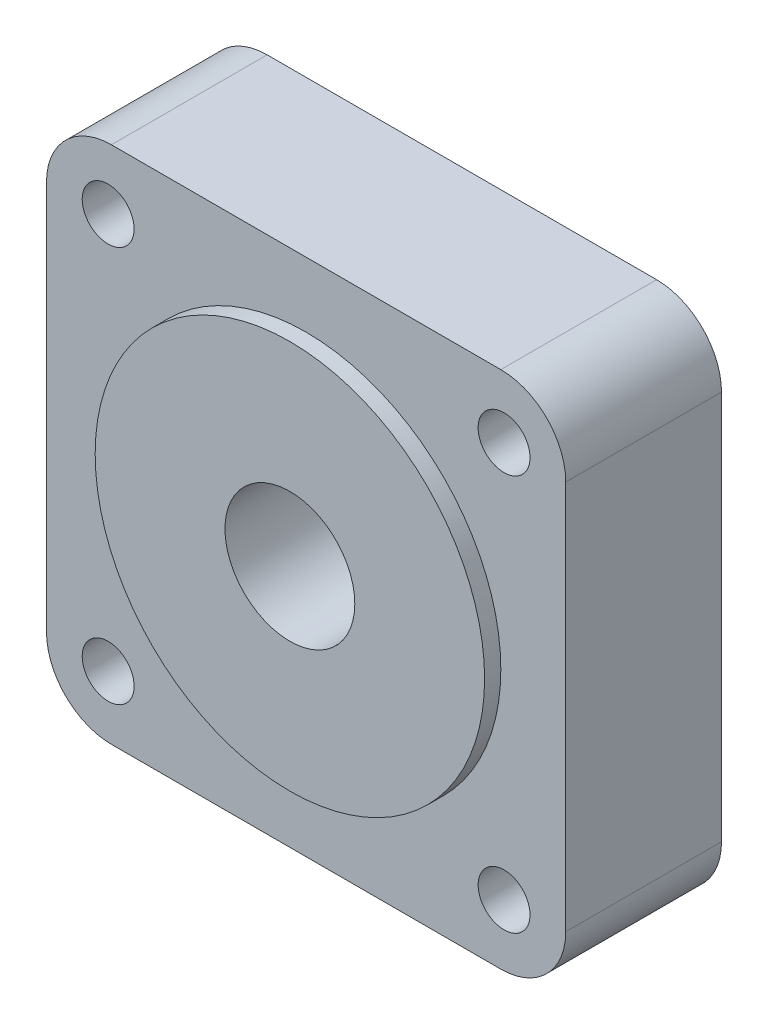
SolidWorks part; units mm, degrees
material "T3"
ref_plane "前视基准面" through (0, 0, 0) normal (0, 0, 1) x (1, 0, 0)
ref_plane "上视基准面" through (0, 0, 0) normal (0, 1, 0) x (1, 0, 0)
ref_plane "右视基准面" through (0, 0, 0) normal (1, 0, 0) x (0, 0, -1)
sketch "草图1" plane through (0, 0, 0) normal (0, 0, 1) x (1, 0, 0)
  line L1 (-40, -40) -> (40, -40)
  line L2 (-40, -40) -> (-40, 40)
  line L3 (-40, 40) -> (40, 40)
  line L4 (40, -40) -> (40, 40)
  line L5 (-40, -40) -> (40, 40) construction
  line L6 (-40, 40) -> (40, -40) construction
  point P0 (0, 0)
  dimension "D1" = 80
  dimension "D2" = 80
extrude "凸台-拉伸1" add sketch "草图1" along normal blind 24
fillet "圆角1" radius 10 4 edges at (-40, -40, 12) (40, -40, 12) (40, 40, 12) (-40, 40, 12)
sketch "草图2" plane through (0, 0, 24) normal (0, 0, 1) x (1, 0, 0)
  line L0 (-37.0711, 37.0711) -> (0, 0) construction
  line L1 (-40, 30) -> (-40, -30) construction
  arc A0 (-30, 40) -> (-40, 30) centre (-30, 30) ccw construction
  circle A1 centre (-30.5, 30.5) radius 4
  dimension "D2" = 8
  dimension "D1" = 9.5
extrude "切除-拉伸1" cut sketch "草图2" against normal through all both and the other way through all
mirror "镜向1" about plane through (0, 0, 0) normal (0, 1, 0) of "切除-拉伸1"
mirror "镜向2" about plane through (0, 0, 0) normal (1, 0, 0) of "镜向1", "切除-拉伸1"
sketch "草图3" plane through (0, 0, 24) normal (0, 0, 1) x (1, 0, 0)
  circle A0 centre (0, 0) radius 30
  dimension "D1" = 60
extrude "凸台-拉伸2" add sketch "草图3" along normal blind 2.5 contours A0
sketch "草图4" plane through (0, 0, 26.5) normal (0, 0, 1) x (1, 0, 0)
  circle A0 centre (0, 0) radius 10
  dimension "D1" = 20
extrude "切除-拉伸2" cut sketch "草图4" against normal blind 49.5
sketch "草图5" plane through (0, 0, 0) normal (0, 0, -1) x (-1, 0, 0)
  line L1 (-23.2635, -25.4385) -> (23.2635, -25.4385)
  line L2 (-25.2635, -23.4385) -> (-25.2635, 23.4385)
  line L3 (-23.2635, 25.4385) -> (23.2635, 25.4385)
  line L4 (25.2635, -23.4385) -> (25.2635, 23.4385)
  line L5 (-25.2635, -25.4385) -> (25.2635, 25.4385) construction
  line L6 (-25.2635, 25.4385) -> (25.2635, -25.4385) construction
  arc A0 (-23.2635, -25.4385) -> (-25.2635, -23.4385) centre (-23.2635, -23.4385) cw
  arc A1 (25.2635, -23.4385) -> (23.2635, -25.4385) centre (23.2635, -23.4385) cw
  arc A2 (25.2635, 23.4385) -> (23.2635, 25.4385) centre (23.2635, 23.4385) ccw
  arc A3 (-25.2635, 23.4385) -> (-23.2635, 25.4385) centre (-23.2635, 23.4385) cw
  point P0 (0, 0)
  dimension "D1" = 2
extrude "切除-拉伸3" cut sketch "草图5" against normal blind 2.5
